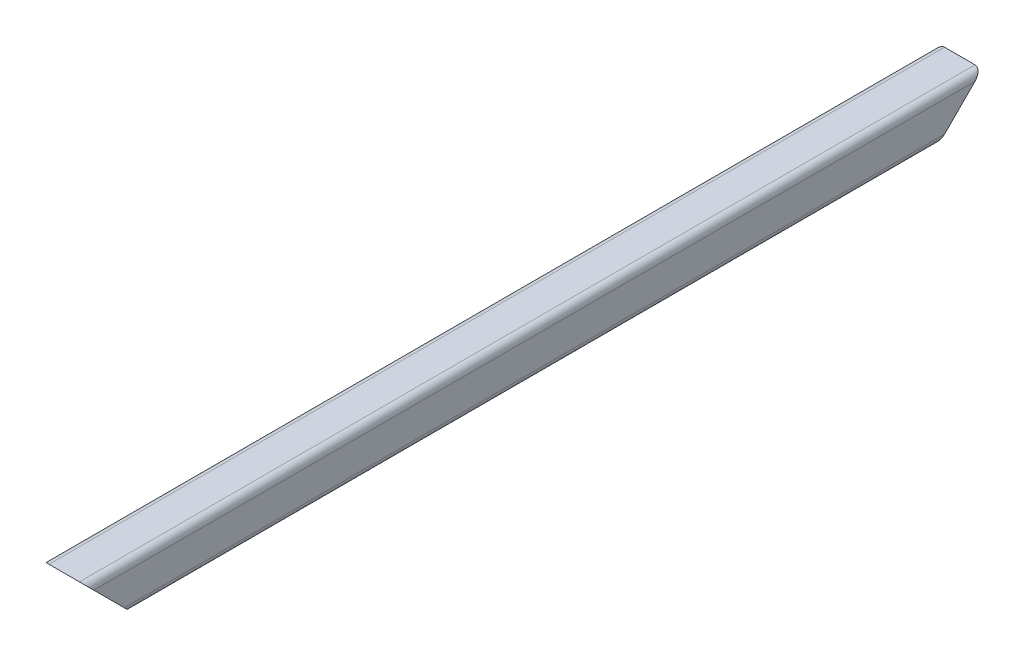
from build123d import *

# Parameters (mm, degrees)
BOSS_EXTRUDE1_DEPTH = 500
CUT_EXTRUDE1_DEPTH  = 504.115294937


with BuildPart() as part:
    # Sketch1 → Boss-Extrude1 (new, symmetric)
    with BuildSketch(Plane.XY):
        with BuildLine():
            Line((-17, -25), (17, -25))
            ThreePointArc((17, -25), (22.656854249, -22.656854249), (25, -17))
            Line((25, -17), (25, 17))
            ThreePointArc((25, 17), (22.656854249, 22.656854249), (17, 25))
            Line((17, 25), (-17, 25))
            ThreePointArc((-17, 25), (-22.656854249, 22.656854249), (-25, 17))
            Line((-25, 17), (-25, -17))
            ThreePointArc((-25, -17), (-22.656854249, -22.656854249), (-17, -25))
        make_face()
        with BuildLine():
            Line((-17, 21), (17, 21))
            ThreePointArc((17, 21), (19.828427125, 19.828427125), (21, 17))
            Line((21, 17), (21, -17))
            ThreePointArc((21, -17), (19.828427125, -19.828427125), (17, -21))
            Line((17, -21), (-17, -21))
            ThreePointArc((-17, -21), (-19.828427125, -19.828427125), (-21, -17))
            Line((-21, -17), (-21, 17))
            ThreePointArc((-21, 17), (-19.828427125, 19.828427125), (-17, 21))
        make_face(mode=Mode.SUBTRACT)
    extrude(amount=BOSS_EXTRUDE1_DEPTH, both=True)

    # Sketch2 → Cut-Extrude1 (cut, through all)
    with BuildSketch(Plane.ZY.offset(25)):
        Polygon((-500, 25), (-450, -25), (-500, -25), align=None)
    cut_extrude1 = extrude(amount=-CUT_EXTRUDE1_DEPTH, mode=Mode.SUBTRACT)

    # Mirror1: Cut-Extrude1 across plane
    add(cut_extrude1.mirror(Plane.XY), mode=Mode.SUBTRACT)


solid = part.part
